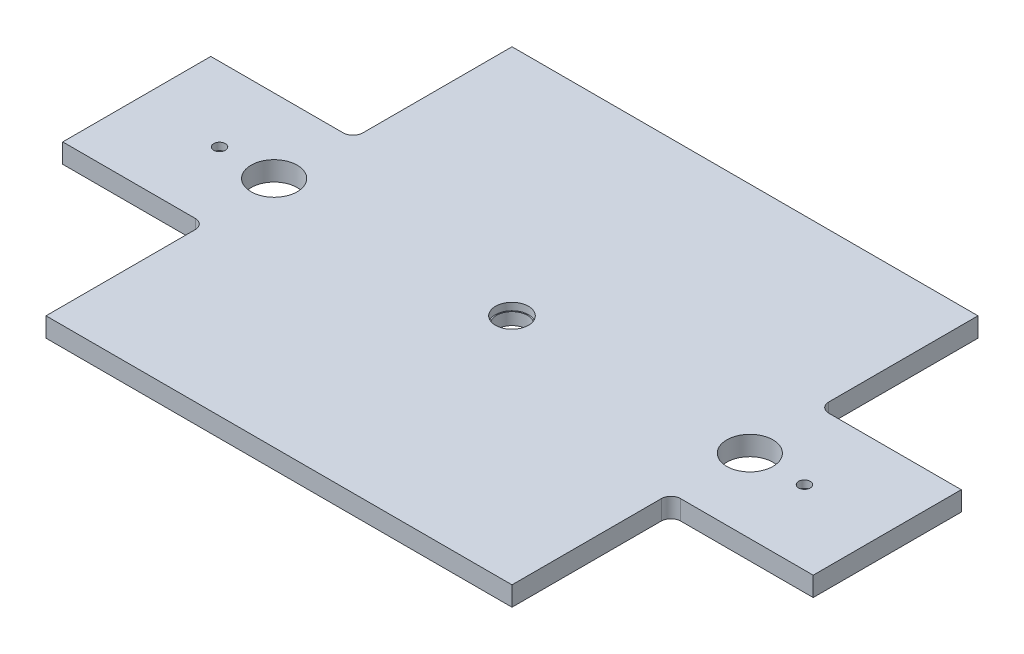
from build123d import *

# Parameters (mm, degrees)
EXTRUDE_1_DEPTH           = 40
SKETCH_2_R                = 20
CUT_EXTRUDE_1_DEPTH       = 10
HOLE_WIZARD_0_D           = 15.5
HOLE_WIZARD_0_CBORE_D     = 24
HOLE_WIZARD_0_CBORE_DEPTH = 15
SKETCH_5_R                = 47.5
CUT_EXTRUDE_2_DEPTH       = 911.7848264
SKETCH_6_R                = 31.75
CUT_EXTRUDE_3_DEPTH       = 911.7848264
FILLET_1_R                = 20
SKETCH_7_R                = 34
CUT_EXTRUDE_4_DEPTH       = 15


with BuildPart() as part:
    # 草图1 → 凸台-拉伸1 (new body)
    with BuildSketch(Plane(origin=(0, 0, 0), x_dir=(1, 0, 0), z_dir=(0, 1, 0))):
        Polygon((-480, 480), (480, 480), (480, 152.5), (773, 152.5), (773, -152.5), (480, -152.5), (480, -480), (-480, -480), (-480, -152.5), (-773, -152.5), (-773, 152.5), (-480, 152.5), align=None)
    extrude(amount=EXTRUDE_1_DEPTH)

    # 草图2 → 切除-拉伸1 (cut)
    with BuildSketch(Plane.XZ):
        with Locations(Location((602.5, 0, 0), (0, 0, 270))):
            Circle(SKETCH_2_R)
    cut_extrude_1 = extrude(amount=-CUT_EXTRUDE_1_DEPTH, mode=Mode.SUBTRACT)

    # 打孔尺寸(%根据)内六角圆柱头螺钉的类型0 (through all)
    with Locations(Plane(origin=(0, 40, 0), x_dir=(1, 0, 0), z_dir=(0, 1, 0))):
        with Locations((602.5, 0)):
            hole_wizard_0 = CounterBoreHole(HOLE_WIZARD_0_D / 2, HOLE_WIZARD_0_CBORE_D / 2, HOLE_WIZARD_0_CBORE_DEPTH)

    # 镜向1: 切除-拉伸1, 打孔尺寸(%根据)内六角圆柱头螺钉的类型0 across plane
    add(cut_extrude_1.mirror(Plane(origin=(0, 0, 0), x_dir=(0, 0, 1), z_dir=(1, 0, 0))), mode=Mode.SUBTRACT)
    add(hole_wizard_0.mirror(Plane(origin=(0, 0, 0), x_dir=(0, 0, 1), z_dir=(1, 0, 0))), mode=Mode.SUBTRACT)

    # 草图5 → 切除-拉伸2 (cut, through all)
    with BuildSketch(Plane.XZ):
        with Locations(Location((490, 0, 0), (0, 0, 270))):
            Circle(SKETCH_5_R)
    cut_extrude_2 = extrude(amount=-CUT_EXTRUDE_2_DEPTH, mode=Mode.SUBTRACT)

    # 镜向2: 切除-拉伸2 across plane
    add(cut_extrude_2.mirror(Plane(origin=(0, 0, 0), x_dir=(0, 0, 1), z_dir=(1, 0, 0))), mode=Mode.SUBTRACT)

    # 草图6 → 切除-拉伸3 (cut, through all)
    with BuildSketch(Plane(origin=(0, 40, 0), x_dir=(1, 0, 0), z_dir=(0, 1, 0))):
        with Locations(Location((0, 0, 0), (0, 0, 270))):
            Circle(SKETCH_6_R)
    extrude(amount=-CUT_EXTRUDE_3_DEPTH, mode=Mode.SUBTRACT)

    # 圆角1
    fillet_1_edges = [part.edges().sort_by_distance(p)[0] for p in [
        (-480, 20, 152.5),
        (-480, 20, -152.5),
        (480, 20, -152.5),
        (480, 20, 152.5),
    ]]
    fillet(fillet_1_edges, radius=FILLET_1_R)

    # 草图7 → 切除-拉伸4 (cut)
    with BuildSketch(Plane(origin=(0, 40, 0), x_dir=(1, 0, 0), z_dir=(0, 1, 0))):
        with Locations(Location((0, 0, 0), (0, 0, 270))):
            Circle(SKETCH_7_R)
    extrude(amount=-CUT_EXTRUDE_4_DEPTH, mode=Mode.SUBTRACT)


solid = part.part
